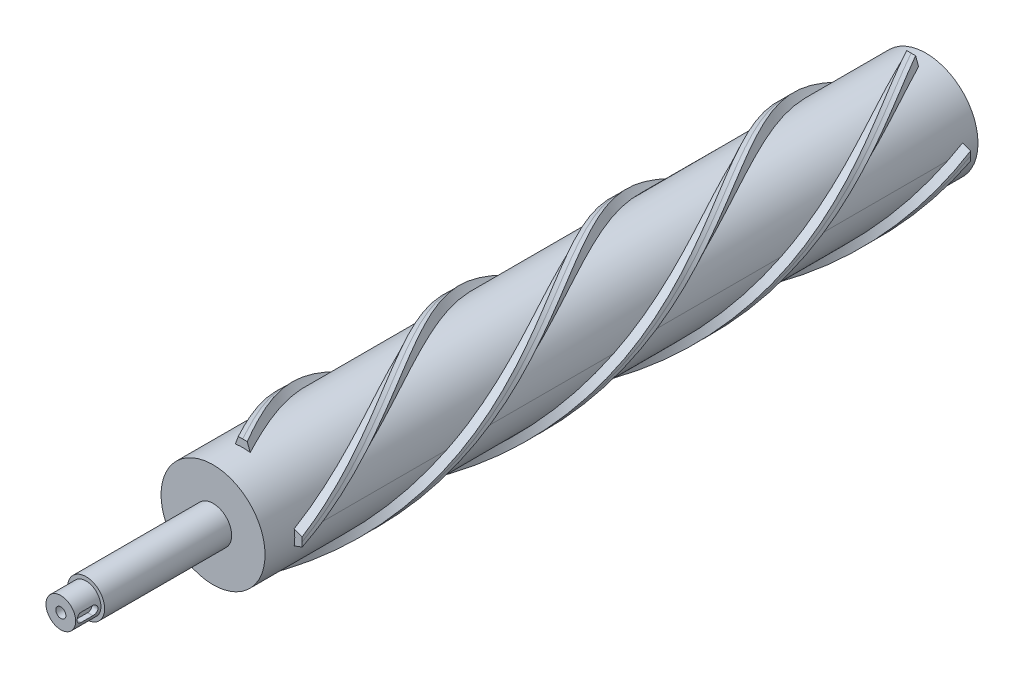
SolidWorks part; units mm, degrees
ref_plane "前视基准面" through (0, 0, 0) normal (0, 0, 1) x (1, 0, 0)
ref_plane "上视基准面" through (0, 0, 0) normal (0, 1, 0) x (1, 0, 0)
ref_plane "右视基准面" through (0, 0, 0) normal (1, 0, 0) x (0, 0, -1)
sketch "草图1" plane through (0, 0, 0) normal (0, 0, 1) x (1, 0, 0)
  circle A0 centre (0, 0) radius 15
extrude "凸台-拉伸1" add sketch "草图1" along normal blind 10
sketch "草图2" plane through (0, 0, 10) normal (0, 0, 1) x (1, 0, 0)
  circle A0 centre (0, 0) radius 35
extrude "凸台-拉伸2" add sketch "草图2" along normal blind 480
sketch "草图3" plane through (0, 0, 490) normal (0, 0, 1) x (1, 0, 0)
  circle A0 centre (0, 0) radius 12.5
extrude "凸台-拉伸3" add sketch "草图3" along normal blind 85.5
ref_plane "基准面1" through (0, 0, 20) normal (0, 0, -1) x (-1, 0, 0)
sketch "草图4" plane through (0, 0, 20) normal (0, 0, -1) x (-1, 0, 0)
  circle A0 centre (0, 0) radius 35
curve "螺旋线/涡状线1" pitch 450 height 450 turns 1
sketch "草图6" plane through (0, 0, 20) normal (0, 0, -1) x (-1, 0, 0)
  line L0 (0, 0) -> (0, 43.7073) construction
  line L1 (-5, 34.641) -> (-5, 32.641)
  line L2 (0, 40) -> (3, 40)
  line L3 (-5, 32.641) -> (5, 32.641)
  line L4 (5, 32.641) -> (5, 34.641)
  line L5 (-3, 40) -> (-5, 34.641)
  line L6 (0, 40) -> (-3, 40)
  line L7 (34.641, 5) -> (32.641, 5)
  line L8 (40, 0) -> (40, -3)
  line L9 (32.641, 5) -> (32.641, -5)
  line L10 (3, 40) -> (5, 34.641)
  line L11 (32.641, -5) -> (34.641, -5)
  line L12 (40, 3) -> (34.641, 5)
  line L13 (40, 0) -> (40, 3)
  line L14 (40, -3) -> (34.641, -5)
  line L15 (5, -34.641) -> (5, -32.641)
  line L16 (0, -40) -> (-3, -40)
  line L17 (5, -32.641) -> (-5, -32.641)
  line L18 (-5, -32.641) -> (-5, -34.641)
  line L19 (3, -40) -> (5, -34.641)
  line L20 (0, -40) -> (3, -40)
  line L21 (-3, -40) -> (-5, -34.641)
  line L22 (-34.641, -5) -> (-32.641, -5)
  line L23 (-40, 0) -> (-40, 3)
  line L24 (-32.641, -5) -> (-32.641, 5)
  line L25 (-32.641, 5) -> (-34.641, 5)
  line L26 (-40, -3) -> (-34.641, -5)
  line L27 (-40, 0) -> (-40, -3)
  line L28 (-40, 3) -> (-34.641, 5)
  point P34 (0, 0)
  dimension "D1" = 4
sweep "扫描1" add profiles "草图6" path "螺旋线/涡状线1"
sketch "草图7" plane through (0, 0, 575.5) normal (0, 0, 1) x (1, 0, 0)
  circle A0 centre (0, 0) radius 10
extrude "凸台-拉伸4" add sketch "草图7" along normal blind 17
ref_plane "基准面2" through (10, 0, 0) normal (1, 0, 0) x (0, 0, -1)
sketch "草图8" plane through (10, 0, 0) normal (1, 0, 0) x (0, 0, -1)
  line L0 (-580.5, 0) -> (-588.5, 0) construction
  line L1 (-575.5, 10) -> (-575.5, -10) construction
  line L2 (-580.5, -3) -> (-588.5, -3)
  line L3 (-580.5, 3) -> (-588.5, 3)
  arc A0 (-580.5, -3) -> (-580.5, 3) centre (-580.5, 0) ccw
  arc A1 (-588.5, 3) -> (-588.5, -3) centre (-588.5, 0) ccw
  point P5 (-584.5, 0)
  dimension "D1" = 8
  dimension "D2" = 3
  dimension "D3" = 5
extrude "切除-拉伸1" cut sketch "草图8" against normal blind 3.96
hole_wizard "M8 螺纹孔1" positions "草图10" profile "草图9" tap size "M8" standard "Iso"
sketch "草图10" plane through (0, 0, 592.5) normal (0, 0, 1) x (1, 0, 0)
  point P0 (0, 0)
sketch "草图9" plane through (0, 0, 592.5) normal (1, 0, 0) x (0, -1, 0)
  line L0 (0, 0) -> (0, 17.0429)
  line L1 (0, 17.0429) -> (3.4, 15)
  line L2 (3.4, 15) -> (3.4, 0)
  line L5 (3.4, 0) -> (0, 0)
  line L10 (0, 17.0429) -> (-3.4, 15) construction
  line L11 (0, -6.35) -> (0, 107.95) construction
  dimension "螺纹孔钻头直径" = 6.8
  dimension "螺纹孔钻头深度" = 15
  dimension "导头角度" = 118
cosmetic thread "孔螺蚊线1" parameters "D1"=15, "D2"=8
